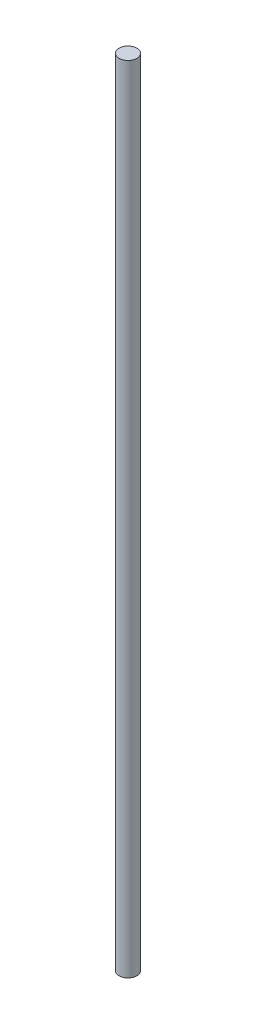
from build123d import *

# Parameters (mm, degrees)
SKETCH1_R           = 125
BOSS_EXTRUDE1_DEPTH = 11200


with BuildPart() as part:
    # Sketch1 → Boss-Extrude1 (new body)
    with BuildSketch(Plane(origin=(0, 0, 0), x_dir=(1, 0, 0), z_dir=(0, 1, 0))):
        with Locations(Location((0, 0, 0), (0, 0, 270))):
            Circle(SKETCH1_R)
    extrude(amount=BOSS_EXTRUDE1_DEPTH)


solid = part.part
